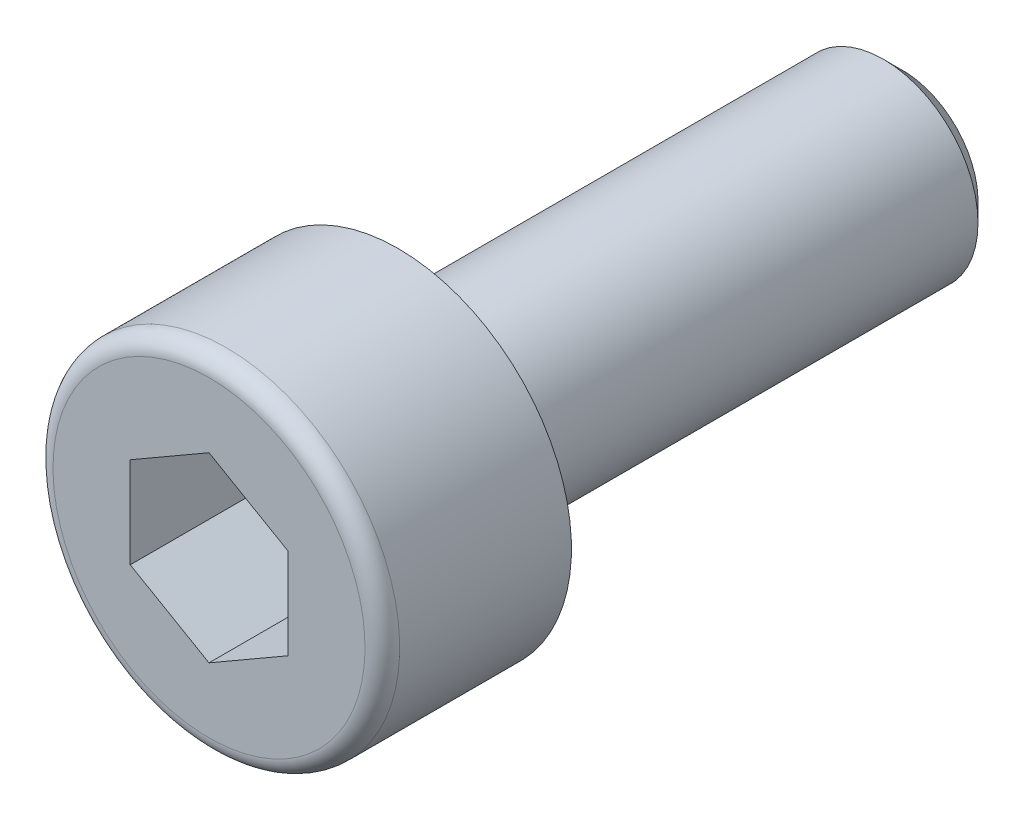
from build123d import *

# Parameters (mm, degrees)
CUT_EXTRUDE_1_DEPTH = 1.925
FILLET_1_R          = 0.275
CHAMFER_1_SIZE      = 0.3


with BuildPart() as part:
    # 草图3 → 旋转1 (revolve)
    with BuildSketch(Plane(origin=(0, 0, 0), x_dir=(0, 0, -1), z_dir=(1, 0, 0)), mode=Mode.PRIVATE) as revolve_1_sk:
        Polygon((-3, 0), (-3, 2.75), (0, 2.75), (0, 1.5), (8, 1.5), (8, 0), align=None)
    revolve(revolve_1_sk.sketch.rotate(Axis((0, 0, 3), (0, 0, -1)), 180), axis=Axis((0, 0, 3), (0, 0, -1)))

    # 草图4 → 切除-拉伸1 (cut)
    with BuildSketch(Plane.XY.offset(3)):
        Polygon((0, 1.443375673), (-1.25, 0.721687836), (-1.25, -0.721687836), (0, -1.443375673), (1.25, -0.721687836), (1.25, 0.721687836), align=None)
    extrude(amount=-CUT_EXTRUDE_1_DEPTH, mode=Mode.SUBTRACT)

    # 圆角1
    fillet_1_edges = [part.edges().sort_by_distance(p)[0] for p in [
        (0, 2.75, 3),
    ]]
    fillet(fillet_1_edges, radius=FILLET_1_R)

    # 倒角1
    chamfer_1_edges = [part.edges().sort_by_distance(p)[0] for p in [
        (0, 1.5, -8),
    ]]
    chamfer(chamfer_1_edges, length=CHAMFER_1_SIZE)


solid = part.part
